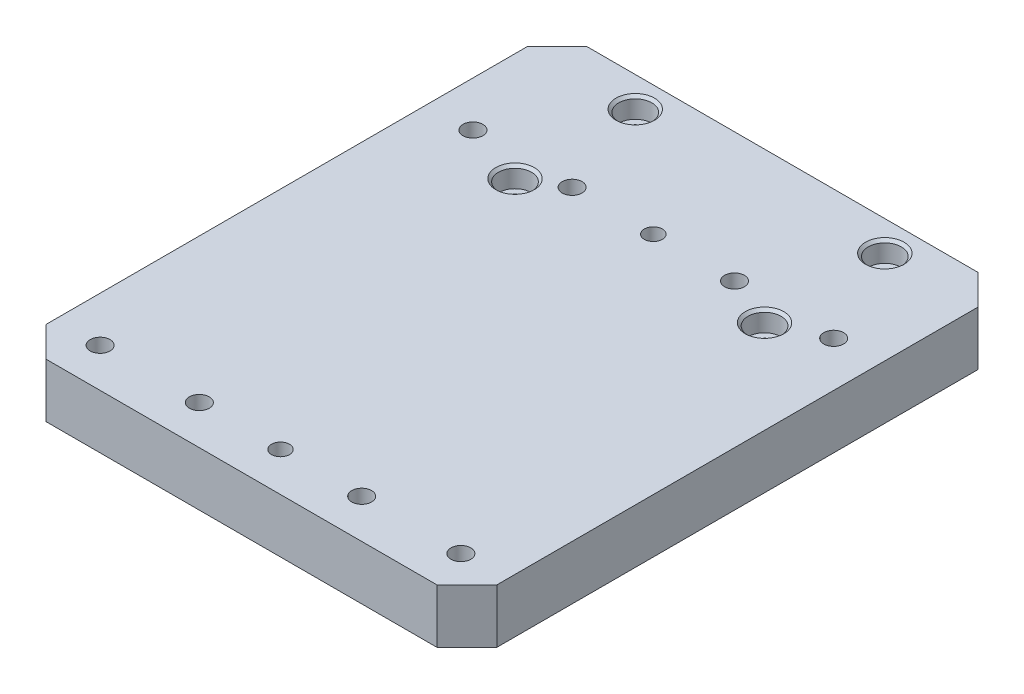
SolidWorks part; units mm, degrees
material "6061 合金"
ref_plane "前视" through (0, 0, 0) normal (0, 0, 1) x (1, 0, 0)
ref_plane "上视" through (0, 0, 0) normal (0, 1, 0) x (1, 0, 0)
ref_plane "右视" through (0, 0, 0) normal (1, 0, 0) x (0, 0, -1)
sketch "草图1" plane through (0, 0, 0) normal (0, 1, 0) x (1, 0, 0)
  line L1 (-75, -90) -> (75, -90)
  line L2 (-75, -90) -> (-75, 90)
  line L3 (-75, 90) -> (75, 90)
  line L4 (75, -90) -> (75, 90)
  line L5 (-75, -90) -> (75, 90) construction
  line L6 (-75, 90) -> (75, -90) construction
  point P0 (0, 0)
  dimension "D1" = 150
  dimension "D2" = 180
extrude "凸台-拉伸1" add sketch "草图1" along normal blind 18
chamfer "倒角1" distance 10 angle 45 4 edges at (-75, 9, -90) (75, 9, -90) (75, 9, 90) (-75, 9, 90)
hole_wizard "打孔尺寸(%根据)内六角圆柱头螺钉的类型1" positions "草图4" profile "草图5" counterbore size "M6" standard "GB" end condition through all
sketch "草图4" plane through (0, 0, 0) normal (0, -1, 0) x (-1, 0, 0)
  point P2 (-60, 47)
  point P5 (-27, 47)
  point P8 (27, 47)
  point P11 (60, 47)
  point P14 (-60, -77)
  point P17 (-27, -77)
  point P20 (27, -77)
  point P23 (60, -77)
sketch "草图5" plane through (60, 0, -47) normal (1, 0, 0) x (0, 0, -1)
  line L0 (0, 0) -> (0, 18)
  line L1 (0, 18) -> (3.3, 18)
  line L3 (3.3, 18) -> (3.3, 6.8)
  line L4 (5.5, 6.8) -> (3.3, 6.8)
  line L5 (5.5, 6.8) -> (5.5, 1.025)
  line L6 (5.5, 1.025) -> (6.525, 0)
  line L7 (6.525, 0) -> (0, 0)
  line L8 (-5.5, 1.025) -> (-6.525, 0) construction
  line L11 (0, -6.35) -> (0, 107.95) construction
  dimension "通孔孔直径" = 6.6
  dimension "通孔孔深度" = 18
  dimension "柱形沉头孔直径" = 11
  dimension "柱形沉头孔深度" = 6.8
  dimension "近端锥形沉头孔直径" = 13.05
  dimension "近端锥形沉头孔角度" = 90
sketch "草图6" plane through (0, 0, 0) normal (0, -1, 0) x (1, 0, 0)
  circle A0 centre (0, -47) radius 3
  circle A1 centre (0, 77) radius 3
extrude "切除-拉伸1" cut sketch "草图6" against normal through all
hole_wizard "打孔尺寸(%根据)内六角圆柱头螺钉的类型2" positions "草图7" profile "草图8" counterbore size "M6" standard "GB" end condition through all
sketch "草图7" plane through (0, 18, 0) normal (0, 1, 0) x (1, 0, 0)
  point P2 (-39, 40)
  point P5 (-39, 80)
  point P8 (44, 80)
  point P11 (44, 40)
sketch "草图8" plane through (-39, 18, -40) normal (1, 0, 0) x (0, 0, 1)
  line L0 (0, 0) -> (0, 18)
  line L1 (0, 18) -> (3.3, 18)
  line L3 (3.3, 18) -> (3.3, 6.8)
  line L4 (5.5, 6.8) -> (3.3, 6.8)
  line L5 (5.5, 6.8) -> (5.5, 0.9)
  line L6 (5.5, 0.9) -> (6.4, 0)
  line L7 (6.4, 0) -> (0, 0)
  line L8 (-5.5, 0.9) -> (-6.4, 0) construction
  line L11 (0, -6.35) -> (0, 107.95) construction
  dimension "通孔孔直径" = 6.6
  dimension "通孔孔深度" = 18
  dimension "柱形沉头孔直径" = 11
  dimension "柱形沉头孔深度" = 6.8
  dimension "近端锥形沉头孔直径" = 12.8
  dimension "近端锥形沉头孔角度" = 90
